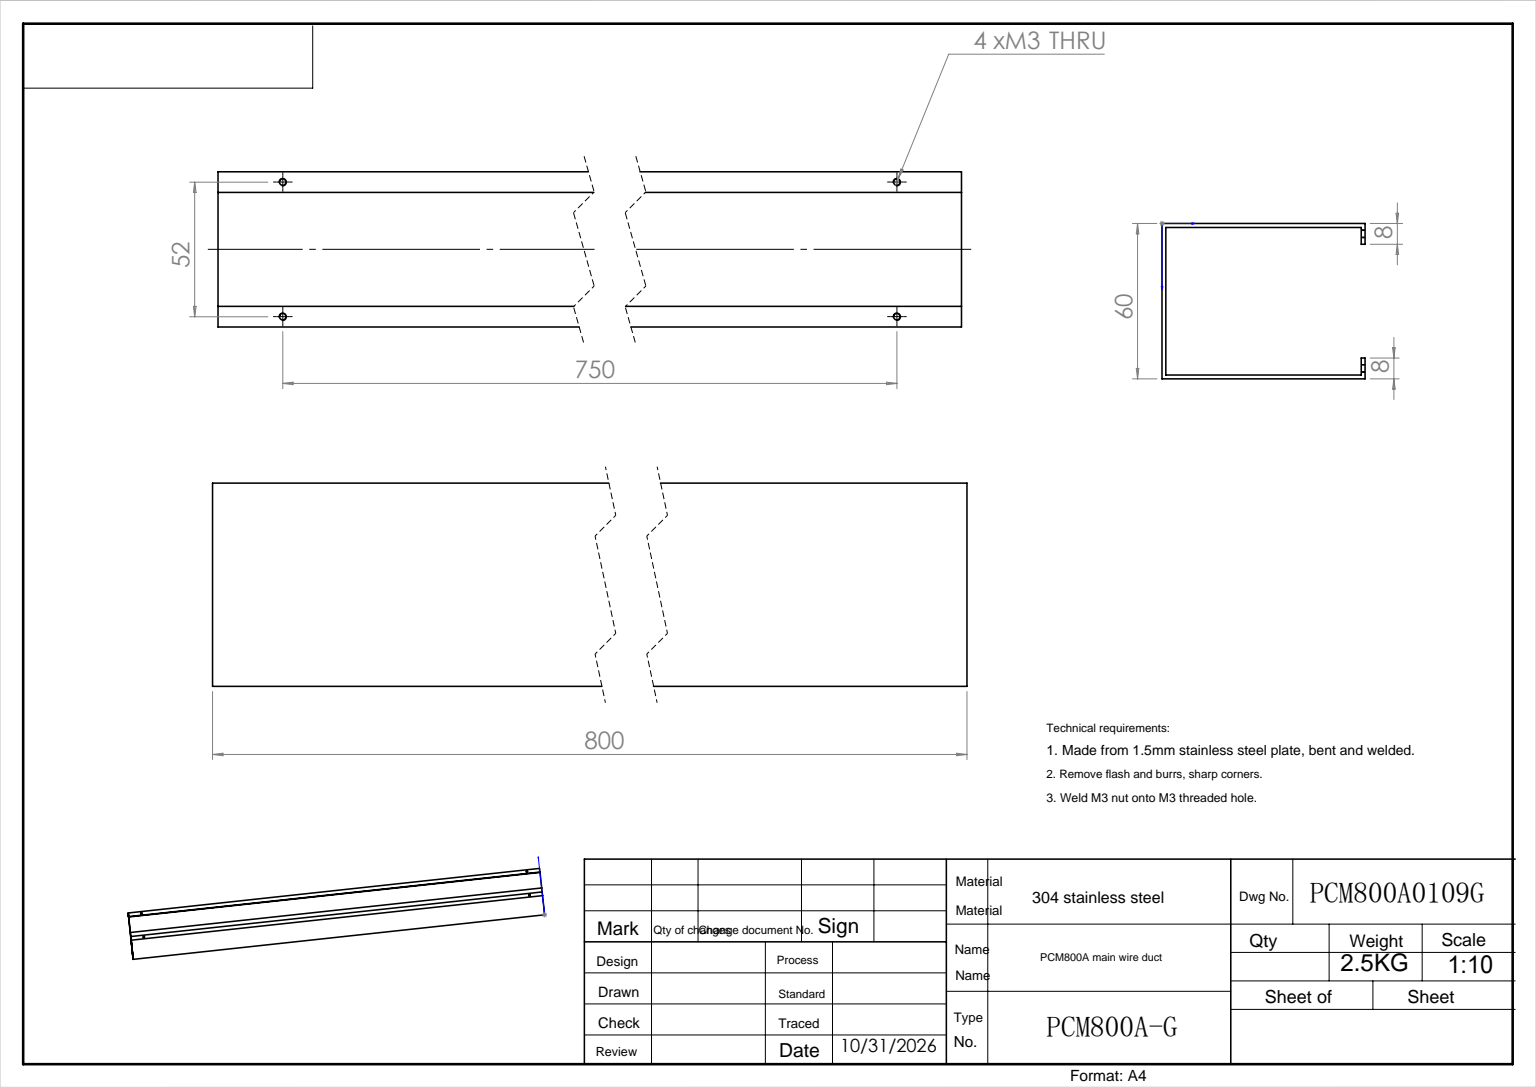
from build123d import *

# Parameters (mm, degrees)
EXTRUDE_1_DEPTH         = 800
HOLE_WIZARD_M3_1_REACH  = 808.078
HOLE_WIZARD_M3_1_BORE_R = 1.25


with BuildPart() as part:
    # 草图1 → 拉伸-薄壁1 (new body)
    with BuildSketch(Plane.XY):
        Polygon((78.5, 52), (78.5, 60), (0, 60), (0, 0), (78.5, 0), (78.5, 8), (77, 8), (77, 1.5), (1.5, 1.5), (1.5, 58.5), (77, 58.5), (77, 52), align=None)
    extrude(amount=EXTRUDE_1_DEPTH)

    # M3 螺纹孔1 bore → M3 螺纹孔1 (cut, up to next)
    with BuildSketch(Plane(origin=(78.5, 0, 0), x_dir=(0, 0, -1), z_dir=(1, 0, 0)), mode=Mode.PRIVATE) as hole_wizard_m3_1_sk1:
        with Locations((-775, 56)):
            Circle(HOLE_WIZARD_M3_1_BORE_R)
    hole_wizard_m3_1_tool1 = extrude(hole_wizard_m3_1_sk1.sketch, amount=-HOLE_WIZARD_M3_1_REACH, mode=Mode.PRIVATE) & part.part
    # M3 螺纹孔1 bore → M3 螺纹孔1 (cut, up to next)
    with BuildSketch(Plane(origin=(78.5, 0, 0), x_dir=(0, 0, -1), z_dir=(1, 0, 0)), mode=Mode.PRIVATE) as hole_wizard_m3_1_sk2:
        with Locations((-25, 56)):
            Circle(HOLE_WIZARD_M3_1_BORE_R)
    hole_wizard_m3_1_tool2 = extrude(hole_wizard_m3_1_sk2.sketch, amount=-HOLE_WIZARD_M3_1_REACH, mode=Mode.PRIVATE) & part.part
    hole_wizard_m3_1_1 = hole_wizard_m3_1_tool1.solids().sort_by_distance((78.5, 56, 775))[0]
    add(hole_wizard_m3_1_1, mode=Mode.SUBTRACT)
    hole_wizard_m3_1_2 = hole_wizard_m3_1_tool2.solids().sort_by_distance((78.5, 56, 25))[0]
    add(hole_wizard_m3_1_2, mode=Mode.SUBTRACT)
    hole_wizard_m3_1 = hole_wizard_m3_1_1 + hole_wizard_m3_1_2  # M3 螺纹孔1 as one shape, for the pattern or mirror that repeats it

    # 镜向2: M3 螺纹孔1 across plane
    add(hole_wizard_m3_1.mirror(Plane(origin=(0, 30, 0), x_dir=(0, 0, 1), z_dir=(0, -1, 0))), mode=Mode.SUBTRACT)


solid = part.part
